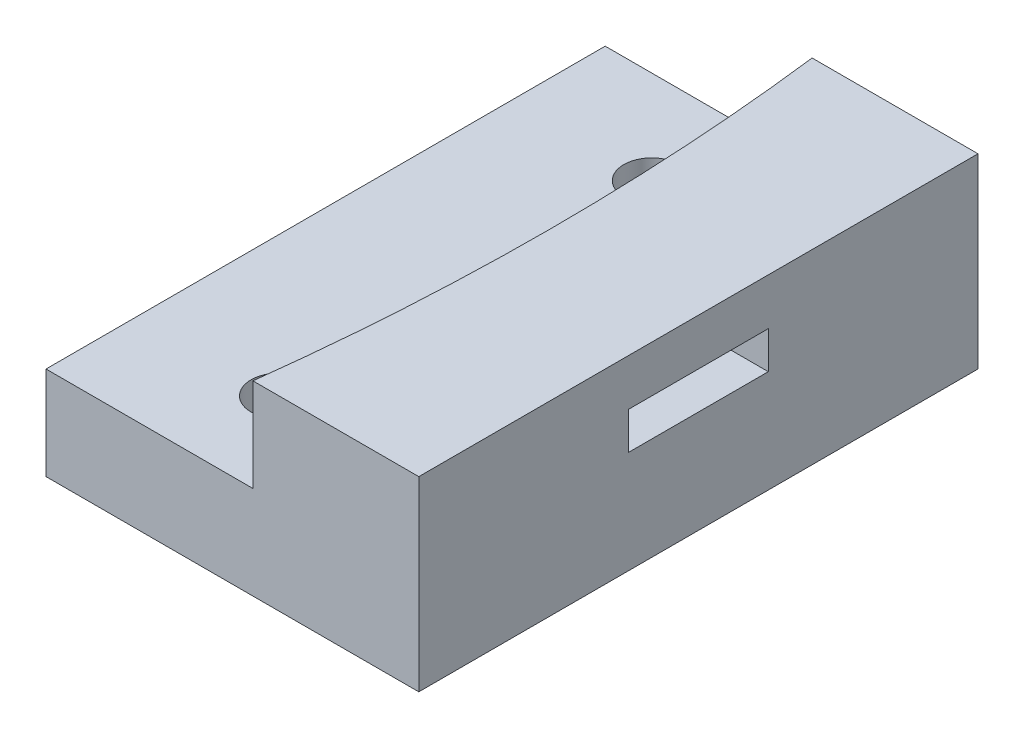
from build123d import *

# Parameters (mm, degrees)
SKETCH1_W           = 40
SKETCH1_H           = 20
BOSS_EXTRUDE1_DEPTH = 60
CUT_EXTRUDE1_DEPTH  = 10
SKETCH3_R           = 3
CUT_EXTRUDE2_DEPTH  = 10
SKETCH4_W           = 15
SKETCH4_H           = 4
CUT_EXTRUDE3_DEPTH  = 49


with BuildPart() as part:
    # Sketch1 → Boss-Extrude1 (new body)
    with BuildSketch(Plane.XY):
        with Locations((20, -10)):
            Rectangle(SKETCH1_W, SKETCH1_H)
    extrude(amount=BOSS_EXTRUDE1_DEPTH)

    # Sketch2 → Cut-Extrude1 (cut)
    with BuildSketch(Plane(origin=(0, 0, 0), x_dir=(1, 0, 0), z_dir=(0, 1, 0))):
        with BuildLine():
            Line((22.2, 0), (0, 0))
            Line((0, 0), (0, -60))
            Line((0, -60), (22.2, -60))
            ThreePointArc((22.2, -60), (24.043671684, -30), (22.2, 0))
        make_face()
    extrude(amount=-CUT_EXTRUDE1_DEPTH, mode=Mode.SUBTRACT)

    # Sketch3 → Cut-Extrude2 (cut)
    with BuildSketch(Plane(origin=(0, -10, 0), x_dir=(1, 0, 0), z_dir=(0, 1, 0))):
        with Locations(Location((15, -10, 0), (0, 0, 270))):
            Circle(SKETCH3_R)
        with Locations(Location((15, -50, 0), (0, 0, 270))):
            Circle(SKETCH3_R)
    extrude(amount=-CUT_EXTRUDE2_DEPTH, mode=Mode.SUBTRACT)

    # Sketch4 → Cut-Extrude3 (cut)
    with BuildSketch(Plane(origin=(40, 0, 0), x_dir=(0, 0, -1), z_dir=(1, 0, 0))):
        with Locations((-30, -7)):
            Rectangle(SKETCH4_W, SKETCH4_H)
    extrude(amount=-CUT_EXTRUDE3_DEPTH, mode=Mode.SUBTRACT)


solid = part.part
